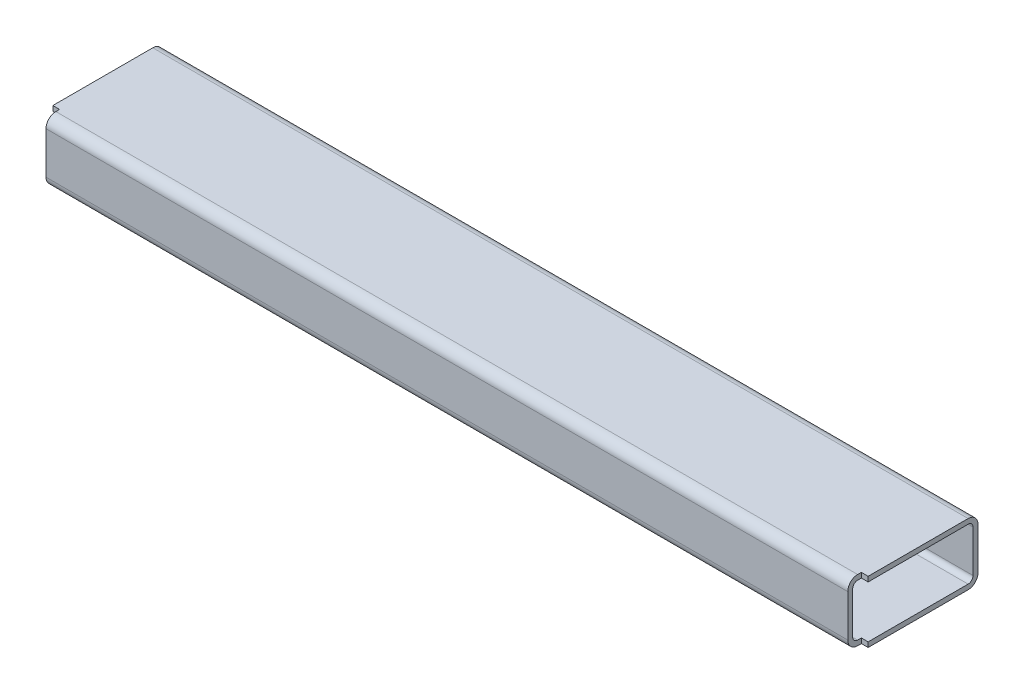
from build123d import *

# Parameters (mm, degrees)
STRUCTURAL_COLD_FORMED_RECTANGULAR_HOLLO_DEPTH = 1321
SKETCH2_W                                      = 11
SKETCH2_H                                      = 22
CUT_EXTRUDE1_DEPTH                             = 676.470391653


with BuildPart() as part:
    # Sketch1 → Structural cold-formed rectangular hollow section (gb t6728-2002) 200×100×8(1) (new body)
    with BuildSketch(Plane.YZ.offset(-660.5)):
        with BuildLine():
            Line((-34, -100), (34, -100))
            ThreePointArc((34, -100), (45.313708499, -95.313708499), (50, -84))
            Line((50, -84), (50, 84))
            ThreePointArc((50, 84), (45.313708499, 95.313708499), (34, 100))
            Line((34, 100), (-34, 100))
            ThreePointArc((-34, 100), (-45.313708499, 95.313708499), (-50, 84))
            Line((-50, 84), (-50, -84))
            ThreePointArc((-50, -84), (-45.313708499, -95.313708499), (-34, -100))
        make_face()
        with BuildLine():
            Line((-34, -92), (34, -92))
            ThreePointArc((34, -92), (39.656854249, -89.656854249), (42, -84))
            Line((42, -84), (42, 84))
            ThreePointArc((42, 84), (39.656854249, 89.656854249), (34, 92))
            Line((34, 92), (-34, 92))
            ThreePointArc((-34, 92), (-39.656854249, 89.656854249), (-42, 84))
            Line((-42, 84), (-42, -84))
            ThreePointArc((-42, -84), (-39.656854249, -89.656854249), (-34, -92))
        make_face(mode=Mode.SUBTRACT)
    extrude(amount=STRUCTURAL_COLD_FORMED_RECTANGULAR_HOLLO_DEPTH)

    # Sketch2 → Cut-Extrude1 (cut, through all)
    with BuildSketch(Plane.XZ.offset(50)):
        with Locations((-655, 89)):
            Rectangle(SKETCH2_W, SKETCH2_H)
    cut_extrude1 = extrude(amount=-CUT_EXTRUDE1_DEPTH, mode=Mode.SUBTRACT)

    # Mirror1: Cut-Extrude1 across plane
    add(cut_extrude1.mirror(Plane(origin=(0, 0, 0), x_dir=(0, 0, 1), z_dir=(1, 0, 0))), mode=Mode.SUBTRACT)


solid = part.part
